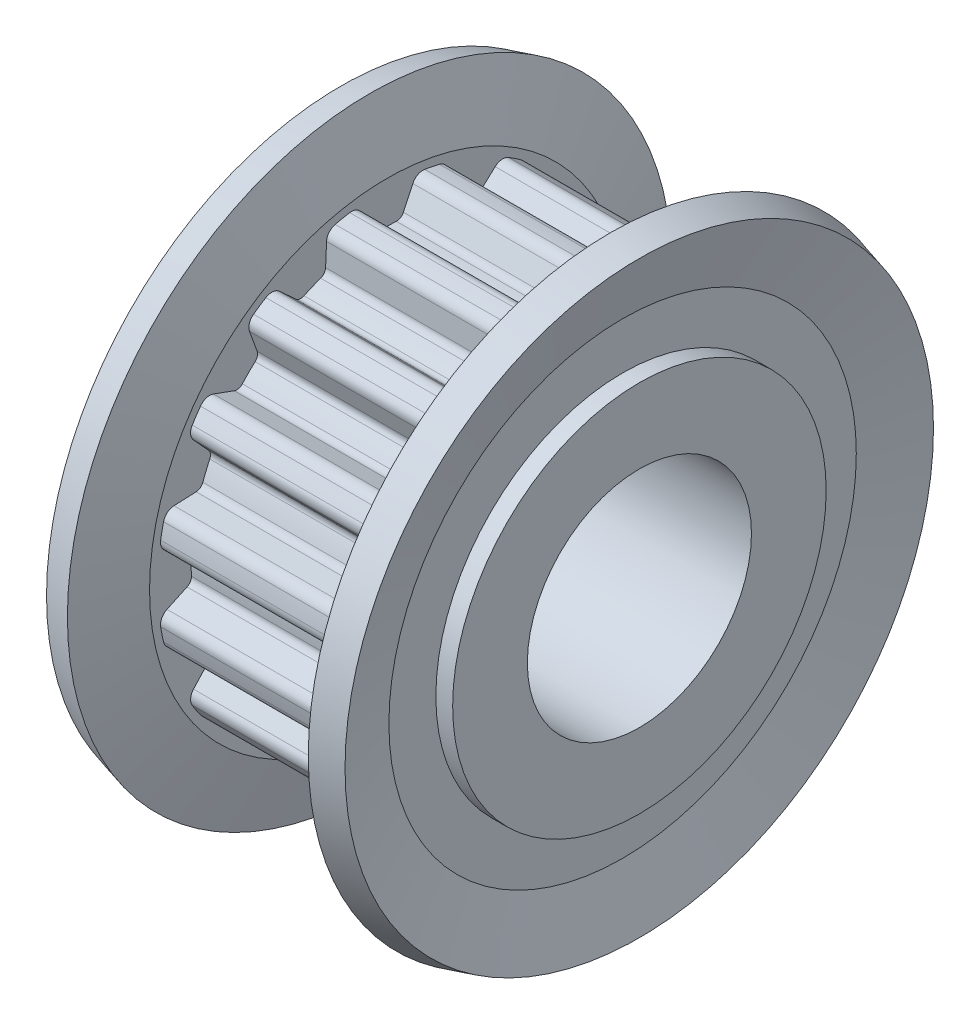
SolidWorks part; units mm, degrees
ref_plane "前视" through (0, 0, 0) normal (0, 0, 1) x (1, 0, 0)
ref_plane "上视" through (0, 0, 0) normal (0, 1, 0) x (1, 0, 0)
ref_plane "右视" through (0, 0, 0) normal (1, 0, 0) x (0, 0, -1)
sketch "草图1" plane through (0, 0, 0) normal (0, 0, 1) x (1, 0, 0)
  line L0 (0, 9.8) -> (0, 6.2)
  line L1 (0, 6.2) -> (0.2, 6)
  line L2 (0.2, 6) -> (16, 6)
  line L3 (16, 6) -> (16, 10)
  line L4 (16, 10) -> (15.1, 10)
  line L5 (15.1, 10) -> (15.1, 12.5138)
  line L6 (15.1, 12.5138) -> (15.9919, 15.7545)
  line L7 (15.9919, 15.7545) -> (14.4493, 16.1791)
  line L8 (14.4493, 16.1791) -> (13.5, 12.73)
  line L9 (13.5, 12.73) -> (2.5, 12.73)
  line L10 (2.5, 12.73) -> (1.5507, 16.1791)
  line L11 (1.5507, 16.1791) -> (0.0081, 15.7545)
  line L12 (0.0081, 15.7545) -> (0.9, 12.5138)
  line L13 (0.9, 12.5138) -> (0.9, 10)
  line L14 (0.9, 10) -> (0.2, 10)
  line L15 (0.2, 10) -> (0, 9.8)
  line L16 (28, 0) -> (0, 0) construction
revolve "旋转1" add sketch "草图1" angle 360 about L16
ref_plane "基准面1" through (2.5, 0, 0) normal (1, 0, 0) x (0, 0, -1)
sketch "草图2" plane through (2.5, 0, 0) normal (1, 0, 0) x (0, 0, -1)
  line L0 (-32, -32) -> (32, -32)
  line L1 (32, -32) -> (32, 32)
  line L2 (32, 32) -> (-32, 32)
  line L3 (-32, 32) -> (-32, -32)
  line L4 (-11.4217, -3.2513) -> (-10.2344, -3.3032)
  line L5 (-9.5725, -4.9011) -> (-10.3754, -5.7773)
  line L6 (-9.308, -7.3747) -> (-8.1912, -6.9682)
  line L7 (-6.9682, -8.1912) -> (-7.3747, -9.308)
  line L8 (-5.7773, -10.3754) -> (-4.9011, -9.5725)
  line L9 (-3.3032, -10.2344) -> (-3.2513, -11.4217)
  line L10 (-1.3671, -11.7965) -> (-0.8648, -10.7194)
  line L11 (0.8648, -10.7194) -> (1.3671, -11.7965)
  line L12 (3.2513, -11.4217) -> (3.3032, -10.2344)
  line L13 (4.9011, -9.5725) -> (5.7773, -10.3754)
  line L14 (7.3747, -9.308) -> (6.9682, -8.1912)
  line L15 (8.1912, -6.9682) -> (9.308, -7.3747)
  line L16 (10.3754, -5.7773) -> (9.5725, -4.9011)
  line L17 (10.2344, -3.3032) -> (11.4217, -3.2513)
  line L18 (11.7965, -1.3671) -> (10.7194, -0.8648)
  line L19 (10.7194, 0.8648) -> (11.7965, 1.3671)
  line L20 (11.4217, 3.2513) -> (10.2344, 3.3032)
  line L21 (9.5725, 4.9011) -> (10.3754, 5.7773)
  line L22 (9.308, 7.3747) -> (8.1912, 6.9682)
  line L23 (6.9682, 8.1912) -> (7.3747, 9.308)
  line L24 (5.7773, 10.3754) -> (4.9011, 9.5725)
  line L25 (3.3032, 10.2344) -> (3.2513, 11.4217)
  line L26 (1.3671, 11.7965) -> (0.8648, 10.7194)
  line L27 (-0.8648, 10.7194) -> (-1.3671, 11.7965)
  line L28 (-3.2513, 11.4217) -> (-3.3032, 10.2344)
  line L29 (-4.9011, 9.5725) -> (-5.7773, 10.3754)
  line L30 (-7.3747, 9.308) -> (-6.9682, 8.1912)
  line L31 (-8.1912, 6.9682) -> (-9.308, 7.3747)
  line L32 (-10.3754, 5.7773) -> (-9.5725, 4.9011)
  line L33 (-10.2344, 3.3032) -> (-11.4217, 3.2513)
  line L34 (-11.7965, 1.3671) -> (-10.7194, 0.8648)
  line L35 (-10.7194, -0.8648) -> (-11.7965, -1.3671)
  arc A0 (-11.7965, -1.3671) -> (-12.1348, -2.0088) centre (-11.5429, -1.9108) ccw
  arc A1 (-12.1348, -2.0088) -> (-12.0637, -2.3996) centre (0, 0) ccw
  arc A2 (-12.0637, -2.3996) -> (-11.9799, -2.7879) centre (0, 0) ccw
  arc A3 (-11.9799, -2.7879) -> (-11.4217, -3.2513) centre (-11.3955, -2.6519) ccw
  arc A4 (-10.2344, -3.3032) -> (-9.8756, -3.5669) centre (-10.2518, -3.7028) cw
  arc A5 (-9.8756, -3.5669) -> (-9.5053, -4.4609) centre (0, 0) ccw
  arc A6 (-9.5053, -4.4609) -> (-9.5725, -4.9011) centre (-9.8674, -4.6309) cw
  arc A7 (-10.3754, -5.7773) -> (-10.4424, -6.4997) centre (-9.933, -6.1827) ccw
  arc A8 (-10.4424, -6.4997) -> (-10.2271, -6.8335) centre (0, 0) ccw
  arc A9 (-10.2271, -6.8335) -> (-10.0011, -7.1602) centre (0, 0) ccw
  arc A10 (-10.0011, -7.1602) -> (-9.308, -7.3747) centre (-9.5132, -6.8109) ccw
  arc A11 (-8.1912, -6.9682) -> (-7.7589, -7.0746) centre (-8.0544, -7.3441) cw
  arc A12 (-7.7589, -7.0746) -> (-7.0746, -7.7589) centre (0, 0) ccw
  arc A13 (-7.0746, -7.7589) -> (-6.9682, -8.1912) centre (-7.3441, -8.0544) cw
  arc A14 (-7.3747, -9.308) -> (-7.1602, -10.0011) centre (-6.8109, -9.5132) ccw
  arc A15 (-7.1602, -10.0011) -> (-6.8335, -10.2271) centre (0, 0) ccw
  arc A16 (-6.8335, -10.2271) -> (-6.4997, -10.4424) centre (0, 0) ccw
  arc A17 (-6.4997, -10.4424) -> (-5.7773, -10.3754) centre (-6.1827, -9.933) ccw
  arc A18 (-4.9011, -9.5725) -> (-4.4609, -9.5053) centre (-4.6309, -9.8674) cw
  arc A19 (-4.4609, -9.5053) -> (-3.5669, -9.8756) centre (0, 0) ccw
  arc A20 (-3.5669, -9.8756) -> (-3.3032, -10.2344) centre (-3.7028, -10.2518) cw
  arc A21 (-3.2513, -11.4217) -> (-2.7879, -11.9799) centre (-2.6519, -11.3955) ccw
  arc A22 (-2.7879, -11.9799) -> (-2.3996, -12.0637) centre (0, 0) ccw
  arc A23 (-2.3996, -12.0637) -> (-2.0088, -12.1348) centre (0, 0) ccw
  arc A24 (-2.0088, -12.1348) -> (-1.3671, -11.7965) centre (-1.9108, -11.5429) ccw
  arc A25 (-0.8648, -10.7194) -> (-0.4838, -10.4888) centre (-0.5023, -10.8884) cw
  arc A26 (-0.4838, -10.4888) -> (0.4838, -10.4888) centre (0, 0) ccw
  arc A27 (0.4838, -10.4888) -> (0.8648, -10.7194) centre (0.5023, -10.8884) cw
  arc A28 (1.3671, -11.7965) -> (2.0088, -12.1348) centre (1.9108, -11.5429) ccw
  arc A29 (2.0088, -12.1348) -> (2.3996, -12.0637) centre (0, 0) ccw
  arc A30 (2.3996, -12.0637) -> (2.7879, -11.9799) centre (0, 0) ccw
  arc A31 (2.7879, -11.9799) -> (3.2513, -11.4217) centre (2.6519, -11.3955) ccw
  arc A32 (3.3032, -10.2344) -> (3.5669, -9.8756) centre (3.7028, -10.2518) cw
  arc A33 (3.5669, -9.8756) -> (4.4609, -9.5053) centre (0, 0) ccw
  arc A34 (4.4609, -9.5053) -> (4.9011, -9.5725) centre (4.6309, -9.8674) cw
  arc A35 (5.7773, -10.3754) -> (6.4997, -10.4424) centre (6.1827, -9.933) ccw
  arc A36 (6.4997, -10.4424) -> (6.8335, -10.2271) centre (0, 0) ccw
  arc A37 (6.8335, -10.2271) -> (7.1602, -10.0011) centre (0, 0) ccw
  arc A38 (7.1602, -10.0011) -> (7.3747, -9.308) centre (6.8109, -9.5132) ccw
  arc A39 (6.9682, -8.1912) -> (7.0746, -7.7589) centre (7.3441, -8.0544) cw
  arc A40 (7.0746, -7.7589) -> (7.7589, -7.0746) centre (0, 0) ccw
  arc A41 (7.7589, -7.0746) -> (8.1912, -6.9682) centre (8.0544, -7.3441) cw
  arc A42 (9.308, -7.3747) -> (10.0011, -7.1602) centre (9.5132, -6.8109) ccw
  arc A43 (10.0011, -7.1602) -> (10.2271, -6.8335) centre (0, 0) ccw
  arc A44 (10.2271, -6.8335) -> (10.4424, -6.4997) centre (0, 0) ccw
  arc A45 (10.4424, -6.4997) -> (10.3754, -5.7773) centre (9.933, -6.1827) ccw
  arc A46 (9.5725, -4.9011) -> (9.5053, -4.4609) centre (9.8674, -4.6309) cw
  arc A47 (9.5053, -4.4609) -> (9.8756, -3.5669) centre (0, 0) ccw
  arc A48 (9.8756, -3.5669) -> (10.2344, -3.3032) centre (10.2518, -3.7028) cw
  arc A49 (11.4217, -3.2513) -> (11.9799, -2.7879) centre (11.3955, -2.6519) ccw
  arc A50 (11.9799, -2.7879) -> (12.0637, -2.3996) centre (0, 0) ccw
  arc A51 (12.0637, -2.3996) -> (12.1348, -2.0088) centre (0, 0) ccw
  arc A52 (12.1348, -2.0088) -> (11.7965, -1.3671) centre (11.5429, -1.9108) ccw
  arc A53 (10.7194, -0.8648) -> (10.4888, -0.4838) centre (10.8884, -0.5023) cw
  arc A54 (10.4888, -0.4838) -> (10.4888, 0.4838) centre (0, 0) ccw
  arc A55 (10.4888, 0.4838) -> (10.7194, 0.8648) centre (10.8884, 0.5023) cw
  arc A56 (11.7965, 1.3671) -> (12.1348, 2.0088) centre (11.5429, 1.9108) ccw
  arc A57 (12.1348, 2.0088) -> (12.0637, 2.3996) centre (0, 0) ccw
  arc A58 (12.0637, 2.3996) -> (11.9799, 2.7879) centre (0, 0) ccw
  arc A59 (11.9799, 2.7879) -> (11.4217, 3.2513) centre (11.3955, 2.6519) ccw
  arc A60 (10.2344, 3.3032) -> (9.8756, 3.5669) centre (10.2518, 3.7028) cw
  arc A61 (9.8756, 3.5669) -> (9.5053, 4.4609) centre (0, 0) ccw
  arc A62 (9.5053, 4.4609) -> (9.5725, 4.9011) centre (9.8674, 4.6309) cw
  arc A63 (10.3754, 5.7773) -> (10.4424, 6.4997) centre (9.933, 6.1827) ccw
  arc A64 (10.4424, 6.4997) -> (10.2271, 6.8335) centre (0, 0) ccw
  arc A65 (10.2271, 6.8335) -> (10.0011, 7.1602) centre (0, 0) ccw
  arc A66 (10.0011, 7.1602) -> (9.308, 7.3747) centre (9.5132, 6.8109) ccw
  arc A67 (8.1912, 6.9682) -> (7.7589, 7.0746) centre (8.0544, 7.3441) cw
  arc A68 (7.7589, 7.0746) -> (7.0746, 7.7589) centre (0, 0) ccw
  arc A69 (7.0746, 7.7589) -> (6.9682, 8.1912) centre (7.3441, 8.0544) cw
  arc A70 (7.3747, 9.308) -> (7.1602, 10.0011) centre (6.8109, 9.5132) ccw
  arc A71 (7.1602, 10.0011) -> (6.8335, 10.2271) centre (0, 0) ccw
  arc A72 (6.8335, 10.2271) -> (6.4997, 10.4424) centre (0, 0) ccw
  arc A73 (6.4997, 10.4424) -> (5.7773, 10.3754) centre (6.1827, 9.933) ccw
  arc A74 (4.9011, 9.5725) -> (4.4609, 9.5053) centre (4.6309, 9.8674) cw
  arc A75 (4.4609, 9.5053) -> (3.5669, 9.8756) centre (0, 0) ccw
  arc A76 (3.5669, 9.8756) -> (3.3032, 10.2344) centre (3.7028, 10.2518) cw
  arc A77 (3.2513, 11.4217) -> (2.7879, 11.9799) centre (2.6519, 11.3955) ccw
  arc A78 (2.7879, 11.9799) -> (2.3996, 12.0637) centre (0, 0) ccw
  arc A79 (2.3996, 12.0637) -> (2.0088, 12.1348) centre (0, 0) ccw
  arc A80 (2.0088, 12.1348) -> (1.3671, 11.7965) centre (1.9108, 11.5429) ccw
  arc A81 (0.8648, 10.7194) -> (0.4838, 10.4888) centre (0.5023, 10.8884) cw
  arc A82 (0.4838, 10.4888) -> (-0.4838, 10.4888) centre (0, 0) ccw
  arc A83 (-0.4838, 10.4888) -> (-0.8648, 10.7194) centre (-0.5023, 10.8884) cw
  arc A84 (-1.3671, 11.7965) -> (-2.0088, 12.1348) centre (-1.9108, 11.5429) ccw
  arc A85 (-2.0088, 12.1348) -> (-2.3996, 12.0637) centre (0, 0) ccw
  arc A86 (-2.3996, 12.0637) -> (-2.7879, 11.9799) centre (0, 0) ccw
  arc A87 (-2.7879, 11.9799) -> (-3.2513, 11.4217) centre (-2.6519, 11.3955) ccw
  arc A88 (-3.3032, 10.2344) -> (-3.5669, 9.8756) centre (-3.7028, 10.2518) cw
  arc A89 (-3.5669, 9.8756) -> (-4.4609, 9.5053) centre (0, 0) ccw
  arc A90 (-4.4609, 9.5053) -> (-4.9011, 9.5725) centre (-4.6309, 9.8674) cw
  arc A91 (-5.7773, 10.3754) -> (-6.4997, 10.4424) centre (-6.1827, 9.933) ccw
  arc A92 (-6.4997, 10.4424) -> (-6.8335, 10.2271) centre (0, 0) ccw
  arc A93 (-6.8335, 10.2271) -> (-7.1602, 10.0011) centre (0, 0) ccw
  arc A94 (-7.1602, 10.0011) -> (-7.3747, 9.308) centre (-6.8109, 9.5132) ccw
  arc A95 (-6.9682, 8.1912) -> (-7.0746, 7.7589) centre (-7.3441, 8.0544) cw
  arc A96 (-7.0746, 7.7589) -> (-7.7589, 7.0746) centre (0, 0) ccw
  arc A97 (-7.7589, 7.0746) -> (-8.1912, 6.9682) centre (-8.0544, 7.3441) cw
  arc A98 (-9.308, 7.3747) -> (-10.0011, 7.1602) centre (-9.5132, 6.8109) ccw
  arc A99 (-10.0011, 7.1602) -> (-10.2271, 6.8335) centre (0, 0) ccw
  arc A100 (-10.2271, 6.8335) -> (-10.4424, 6.4997) centre (0, 0) ccw
  arc A101 (-10.4424, 6.4997) -> (-10.3754, 5.7773) centre (-9.933, 6.1827) ccw
  arc A102 (-9.5725, 4.9011) -> (-9.5053, 4.4609) centre (-9.8674, 4.6309) cw
  arc A103 (-9.5053, 4.4609) -> (-9.8756, 3.5669) centre (0, 0) ccw
  arc A104 (-9.8756, 3.5669) -> (-10.2344, 3.3032) centre (-10.2518, 3.7028) cw
  arc A105 (-11.4217, 3.2513) -> (-11.9799, 2.7879) centre (-11.3955, 2.6519) ccw
  arc A106 (-11.9799, 2.7879) -> (-12.0637, 2.3996) centre (0, 0) ccw
  arc A107 (-12.0637, 2.3996) -> (-12.1348, 2.0088) centre (0, 0) ccw
  arc A108 (-12.1348, 2.0088) -> (-11.7965, 1.3671) centre (-11.5429, 1.9108) ccw
  arc A109 (-10.7194, 0.8648) -> (-10.4888, 0.4838) centre (-10.8884, 0.5023) cw
  arc A110 (-10.4888, 0.4838) -> (-10.4888, -0.4838) centre (0, 0) ccw
  arc A111 (-10.4888, -0.4838) -> (-10.7194, -0.8648) centre (-10.8884, -0.5023) cw
extrude "切除-拉伸1" cut sketch "草图2" along normal blind 11
ref_plane "基准面2" through (8, 0, 0) normal (1, 0, 0) x (0, 0, -1)
